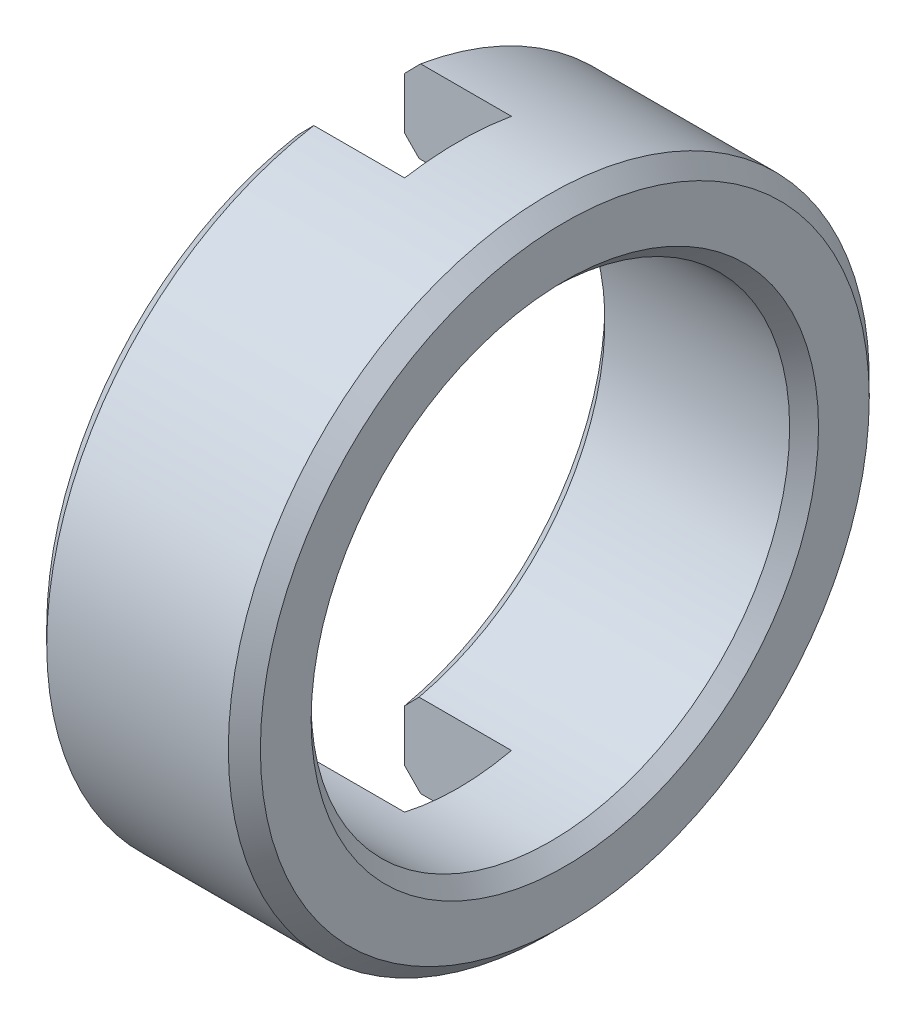
from build123d import *

# Parameters (mm, degrees)
CUT_EXTRUDE_1_DEPTH      = 1
CUT_EXTRUDE_1_DEPTH_BACK = 1
SKETCH_2_W               = 5
SKETCH_2_H               = 20


with BuildPart() as part:
    # 草图1 → 旋转1 (revolve)
    with BuildSketch(Plane.XY, mode=Mode.PRIVATE) as revolve_1_sk:
        Polygon((-2, 4.75), (-1.7295, 4.4795), (1.7295, 4.4795), (2, 4.75), (2, 5.7), (1.7, 6), (-1.7, 6), (-2, 5.7), align=None)
    revolve(revolve_1_sk.sketch.rotate(Axis((2, 0, 0), (-1, 0, 0)), 270), axis=Axis((2, 0, 0), (-1, 0, 0)))

    # 草图2 → 切除-拉伸1 (cut, two sides: drawn at the far end of the back side and taken through both)
    with BuildSketch(Plane.XY.offset(-CUT_EXTRUDE_1_DEPTH_BACK)):
        with Locations((-2.5, 0)):
            Rectangle(SKETCH_2_W, SKETCH_2_H)
    extrude(amount=CUT_EXTRUDE_1_DEPTH + CUT_EXTRUDE_1_DEPTH_BACK, mode=Mode.SUBTRACT)


solid = part.part
